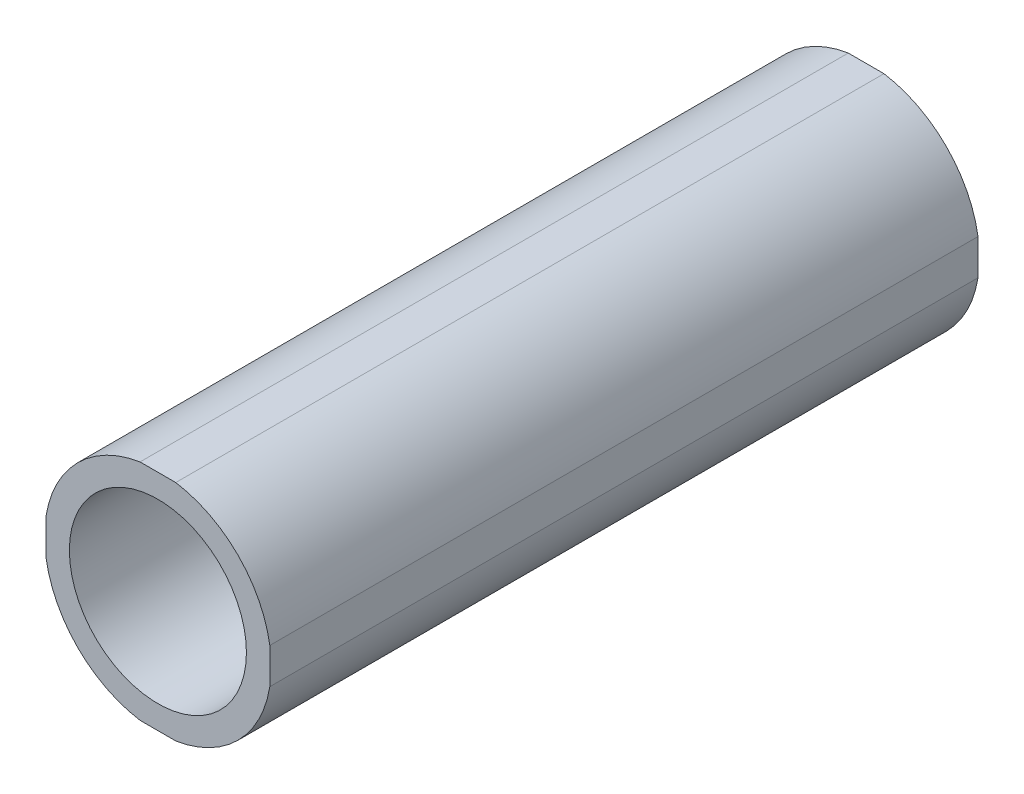
from build123d import *

# Parameters (mm, degrees)
SKETCH1_R           = 8
SKETCH1_R_2         = 6.25
BOSS_EXTRUDE1_DEPTH = 50
SKETCH2_W           = 20.877121254
SKETCH2_H           = 20.159055414
SKETCH2_W_2         = 15.8
SKETCH2_H_2         = 15.8
CUT_EXTRUDE1_DEPTH  = 50


with BuildPart() as part:
    # Sketch1 → Boss-Extrude1 (new body)
    with BuildSketch(Plane.XY):
        Circle(SKETCH1_R)
        Circle(SKETCH1_R_2, mode=Mode.SUBTRACT)
    extrude(amount=BOSS_EXTRUDE1_DEPTH)

    # Sketch2 → Cut-Extrude1 (cut)
    with BuildSketch(Plane.XY.offset(50)):
        Rectangle(SKETCH2_W, SKETCH2_H)
        Rectangle(SKETCH2_W_2, SKETCH2_H_2, mode=Mode.SUBTRACT)
    extrude(amount=-CUT_EXTRUDE1_DEPTH, mode=Mode.SUBTRACT)


solid = part.part
